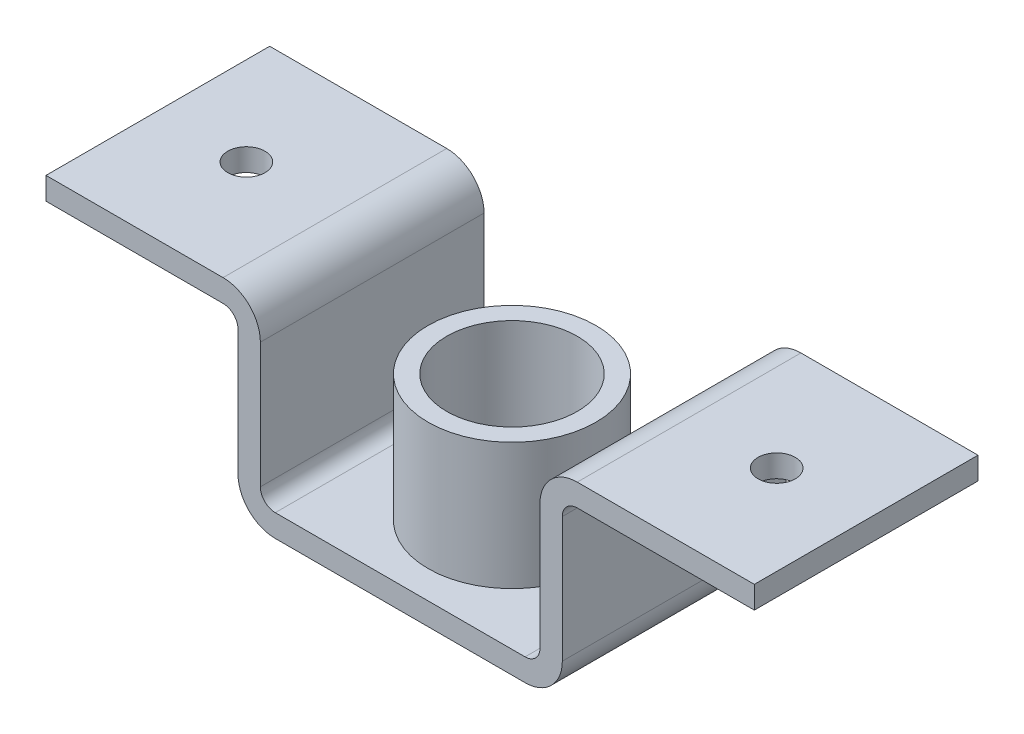
from build123d import *

# Parameters (mm, degrees)
BOSS_EXTRUDE2_DEPTH = 300
FILLET3_R           = 20
FILLET4_R           = 50
FILLET5_R           = 20
SKETCH2_R           = 112.5
SKETCH2_R_2         = 87.5
BOSS_EXTRUDE3_DEPTH = 170
CUT_EXTRUDE1_REACH  = 612.139
SKETCH3_R           = 37.5
CUT_EXTRUDE2_REACH  = 624.454
SKETCH4_R           = 25


with BuildPart() as part:
    # Sketch1 → Boss-Extrude2 (new body)
    with BuildSketch(Plane.XY):
        Polygon((187.5, 0), (-187.5, 0), (-187.5, 238), (-475, 238), (-475, 208), (-217.5, 208), (-217.5, -30), (217.5, -30), (217.5, 208), (475, 208), (475, 238), (187.5, 238), align=None)
    extrude(amount=BOSS_EXTRUDE2_DEPTH)

    # Fillet3
    fillet3_edges = [part.edges().sort_by_distance(p)[0] for p in [
        (-187.5, 0, 150),
        (187.5, 0, 150),
    ]]
    fillet(fillet3_edges, radius=FILLET3_R)

    # Fillet4
    fillet4_edges = [part.edges().sort_by_distance(p)[0] for p in [
        (187.5, 238, 150),
        (217.5, -30, 150),
        (-217.5, -30, 150),
        (-187.5, 238, 150),
    ]]
    fillet(fillet4_edges, radius=FILLET4_R)

    # Fillet5
    fillet5_edges = [part.edges().sort_by_distance(p)[0] for p in [
        (217.5, 208, 150),
        (-217.5, 208, 150),
    ]]
    fillet(fillet5_edges, radius=FILLET5_R)

    # Sketch2 → Boss-Extrude3 (add)
    with BuildSketch(Plane(origin=(0, 0, 0), x_dir=(1, 0, 0), z_dir=(0, 1, 0))):
        with Locations((0, -150)):
            Circle(SKETCH2_R)
        with Locations(Location((0, -150, 0), (0, 0, 180))):
            Circle(SKETCH2_R_2, mode=Mode.SUBTRACT)
    extrude(amount=BOSS_EXTRUDE3_DEPTH)

    # Sketch3 → Cut-Extrude1 (cut, up to next)
    with BuildSketch(Plane(origin=(0, 0, 0), x_dir=(1, 0, 0), z_dir=(0, 1, 0)), mode=Mode.PRIVATE) as cut_extrude1_sk1:
        with Locations(Location((0, -150, 0), (0, 0, 180))):
            Circle(SKETCH3_R)
    cut_extrude1_tool1 = extrude(cut_extrude1_sk1.sketch, amount=-CUT_EXTRUDE1_REACH, mode=Mode.PRIVATE) & part.part
    add(cut_extrude1_tool1.solids().sort_by_distance((0, 0, 150))[0], mode=Mode.SUBTRACT)

    # Sketch4 → Cut-Extrude2 (cut, up to next)
    with BuildSketch(Plane(origin=(0, 238, 0), x_dir=(1, 0, 0), z_dir=(0, 1, 0)), mode=Mode.PRIVATE) as cut_extrude2_sk1:
        with Locations(Location((-356.25, -150, 0), (0, 0, 180))):
            Circle(SKETCH4_R)
    cut_extrude2_tool1 = extrude(cut_extrude2_sk1.sketch, amount=-CUT_EXTRUDE2_REACH, mode=Mode.PRIVATE) & part.part
    # Sketch4 → Cut-Extrude2 (cut, up to next)
    with BuildSketch(Plane(origin=(0, 238, 0), x_dir=(1, 0, 0), z_dir=(0, 1, 0)), mode=Mode.PRIVATE) as cut_extrude2_sk2:
        with Locations(Location((355, -150, 0), (0, 0, 180))):
            Circle(SKETCH4_R)
    cut_extrude2_tool2 = extrude(cut_extrude2_sk2.sketch, amount=-CUT_EXTRUDE2_REACH, mode=Mode.PRIVATE) & part.part
    add(cut_extrude2_tool1.solids().sort_by_distance((-356.25, 238, 150))[0], mode=Mode.SUBTRACT)
    add(cut_extrude2_tool2.solids().sort_by_distance((355, 238, 150))[0], mode=Mode.SUBTRACT)


solid = part.part
